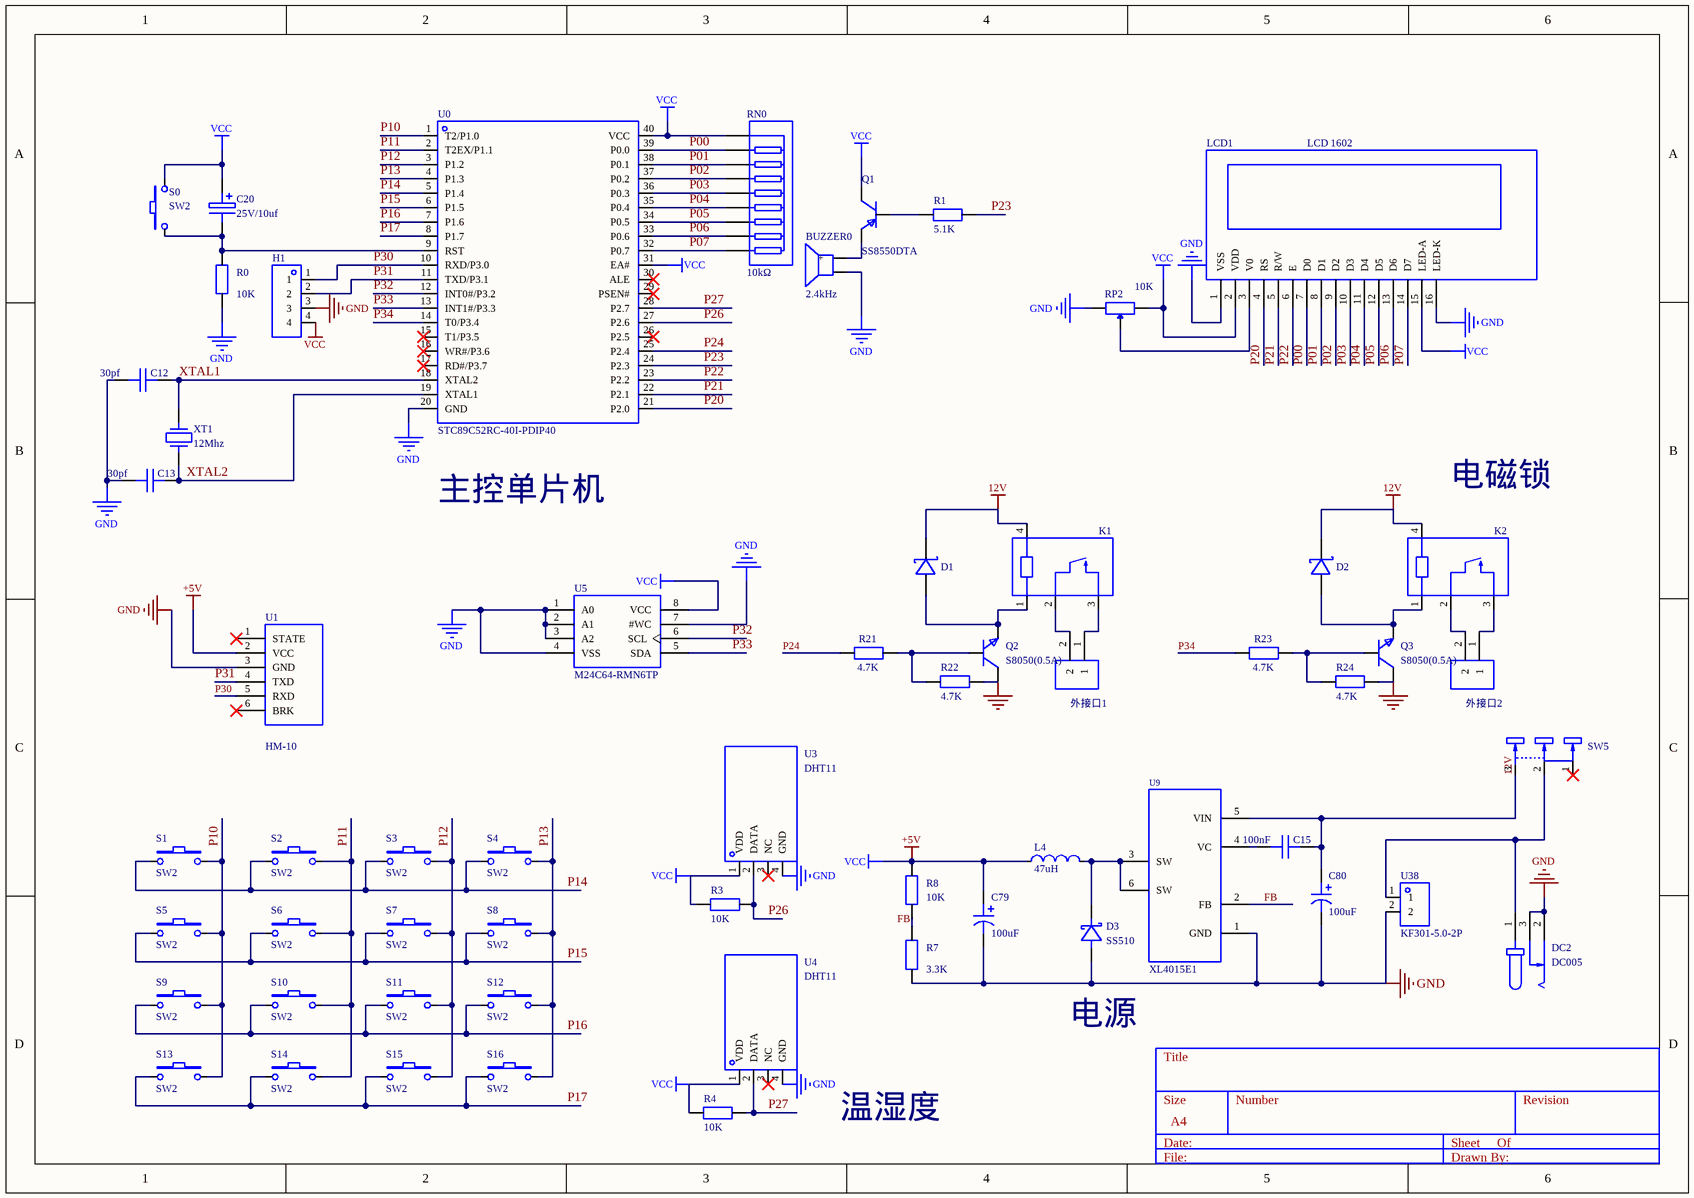
[diagram p0: MISC52141-3.schdoc]
# Altium project MISC52141-2.PrjPcb
1 sheet, 59 parts. Net scope: global (net labels, ports and power ports of the same name join across sheets).
Board file: MISC52141.pcbdoc

## Sheet MISC52141-3.schdoc
size 297 x 209 mm

### Parts
BUZZER0  2.4kHz  [BUZ-TH_BD12.0-P7.60-D0.6-FD]
C12  30pf  [C0805]
C13  30pf  [C0805]
C15  100nF  [C0805]
C20  value 25V/10uf  [CAP-TH_BD5.0-P2.00-D0.5-FD-A]  (hidden comment: CAP-E)
C79  100uF  [CAP-SMD_BD6.3-L6.6-W6.6-LS7.4-FD]
C80  100uF  [CAP-SMD_BD6.3-L6.6-W6.6-LS7.4-FD]
D1  (no value)  [SMC_L6.9-W5.9-LS7.9-RD]
D2  (no value)  [SMC_L6.9-W5.9-LS7.9-RD]
D3  SS510  [SMA_L4.3-W2.6-LS5.0-RD]
DC2  DC005  [DC-IN-TH_DC005]
H1  (no value)  [HDR-TH_4P-P2.54-V-F]
K1  (no value)  [RELAY-TH_G5NB-1A-E-DCXX]
K2  (no value)  [RELAY-TH_G5NB-1A-E-DCXX]
L4  47uH  [IND-SMD_L12.3-W12.3]
LCD1  LCD 1602  [LCD1602]
Q1  SS8550DTA  [TO-92-3_L4.8-W3.7-P2.54-L]
Q2  S8050(0.5A)  [SOT-23-3_L2.9-W1.3-P1.90-LS2.4-BR]
Q3  S8050(0.5A)  [SOT-23-3_L2.9-W1.3-P1.90-LS2.4-BR]
R0  10K  [R0805]
R1  5.1K  [R0805]
R3  10K  [R0805]
R4  10K  [R0805]
R7  3.3K  [R0805]
R8  10K  [R0805]
R21  4.7K  [R0805]
R22  4.7K  [R0805]
R23  4.7K  [R0805]
R24  4.7K  [R0805]
RN0  10kΩ  [RES-ARRAY-TH_9P-P2.54-D1.0]
RP2  10K  [RES-ADJ-TH_3296W-1-203]
S0  SW2  [SW-SMD_L3.9-W2.9-LS5.0]
S1  SW2  [SW-SMD_L3.9-W2.9-LS5.0]
S2  SW2  [SW-SMD_L3.9-W2.9-LS5.0]
S3  SW2  [SW-SMD_L3.9-W2.9-LS5.0]
S4  SW2  [SW-SMD_L3.9-W2.9-LS5.0]
S5  SW2  [SW-SMD_L3.9-W2.9-LS5.0]
S6  SW2  [SW-SMD_L3.9-W2.9-LS5.0]
S7  SW2  [SW-SMD_L3.9-W2.9-LS5.0]
S8  SW2  [SW-SMD_L3.9-W2.9-LS5.0]
S9  SW2  [SW-SMD_L3.9-W2.9-LS5.0]
S10  SW2  [SW-SMD_L3.9-W2.9-LS5.0]
S11  SW2  [SW-SMD_L3.9-W2.9-LS5.0]
S12  SW2  [SW-SMD_L3.9-W2.9-LS5.0]
S13  SW2  [SW-SMD_L3.9-W2.9-LS5.0]
S14  SW2  [SW-SMD_L3.9-W2.9-LS5.0]
S15  SW2  [SW-SMD_L3.9-W2.9-LS5.0]
S16  SW2  [SW-SMD_L3.9-W2.9-LS5.0]
SW5  SS-12D10L5  [SW-TH_SS-12D10L5]  (value not drawn)
U0  STC89C52RC-40I-PDIP40  [DIP-40_L52.0-W13.7-P2.54-LS15.2-BL]
U1  HM-10  [HM-10.288]
U3  DHT11  [SENSOR-TH_DHT11]
U4  DHT11  [SENSOR-TH_DHT11]
U5  M24C64-RMN6TP  [SOIC-8_L5.0-W4.0-P1.27-LS6.0-BL]
U9  XL4015E1  [TO-263-5_L10.2-W8.9-P1.70-TL]
U38  KF301-5.0-2P  [CONN-TH_P5.00_KF301-5.0-2P]
XT1  value 12Mhz  [HC-49S_L7.2-W3.2]  (hidden comment: XT)
外接口1  (no value)  [CONN-TH_2P-P5.00_WJ500V-5.08-2P]
外接口2  (no value)  [CONN-TH_2P-P5.00_WJ500V-5.08-2P]

### Nets
12V: C15.1 C80.1 D1.1(C) D2.1(C) K1.4 K2.4 SW5.3 U9.5(VIN)
+5V: C20.1 C79.1 H1.4 L4.1 LCD1.2(VDD) LCD1.15(LED-A) Q1.3(C) R3.2 R4.2 R8.2 RN0.1 RP2.1 S0.2 U0.31(EA#) U0.40(VCC) U1.2(VCC) U3.1(VDD) U4.1(VDD) U5.8(VCC)  [also labelled VCC]
GND: BUZZER0.2 C12.2 C13.2 C79.2 C80.2 D3.2(A) DC2.2 DC2.3 H1.3 LCD1.1(VSS) LCD1.16(LED-K) Q2.3(C) Q3.3(C) R0.1 R7.1 R22.1 R24.1 RP2.3 U0.20(GND) U1.3(GND) U3.4(GND) U4.4(GND) U5.1(A0) U5.2(A1) U5.3(A2) U5.4(VSS) U5.7(#WC) U9.1(GND) U38.2
FB: R7.2 R8.1 U9.2(FB)
P00: LCD1.7(D0) RN0.2 U0.39(P0.0)
P01: LCD1.8(D1) RN0.3 U0.38(P0.1)
P02: LCD1.9(D2) RN0.4 U0.37(P0.2)
P03: LCD1.10(D3) RN0.5 U0.36(P0.3)
P04: LCD1.11(D4) RN0.6 U0.35(P0.4)
P05: LCD1.12(D5) RN0.7 U0.34(P0.5)
P06: LCD1.13(D6) RN0.8 U0.33(P0.6)
P07: LCD1.14(D7) RN0.9 U0.32(P0.7)
P10: S1.2 S5.2 S9.2 S13.2 U0.1(T2/P1.0)
P11: S2.2 S6.2 S10.2 S14.2 U0.2(T2EX/P1.1)
P12: S3.2 S7.2 S11.2 S15.2 U0.3(P1.2)
P13: S4.2 S8.2 S12.2 S16.2 U0.4(P1.3)
P14: S1.1 S2.1 S3.1 S4.1 U0.5(P1.4)
P15: S5.1 S6.1 S7.1 S8.1 U0.6(P1.5)
P16: S9.1 S10.1 S11.1 S12.1 U0.7(P1.6)
P17: S13.1 S14.1 S15.1 S16.1 U0.8(P1.7)
P20: LCD1.4(RS) U0.21(P2.0)
P21: LCD1.5(R/W) U0.22(P2.1)
P22: LCD1.6(E) U0.23(P2.2)
P23: R1.1 U0.24(P2.3)
P24: R21.2 U0.25(P2.4)
P26: R3.1 U0.27(P2.6) U3.2(DATA)
P27: R4.1 U0.28(P2.7) U4.2(DATA)
P30: H1.1 U0.10(RXD/P3.0) U1.5(RXD)
P31: H1.2 U0.11(TXD/P3.1) U1.4(TXD)
P32: U0.12(INT0#/P3.2) U5.6(SCL)
P33: U0.13(INT1#/P3.3) U5.5(SDA)
P34: R23.2 U0.14(T0/P3.4)
XTAL1: C12.1 U0.18(XTAL2) XT1.2
XTAL2: C13.1 U0.19(XTAL1) XT1.1
NetBUZZER0_1: BUZZER0.1(+) Q1.1(E)
NetC15_2: C15.2 U9.4(VC)
NetC20_2: C20.2 R0.2 S0.1 U0.9(RST)
NetD1_2: D1.2(A) K1.1 Q2.2(E)
NetD2_2: D2.2(A) K2.1 Q3.2(E)
NetD3_1: D3.1(K) L4.2 U9.3(SW) U9.6(SW)
NetDC2_1: DC2.1 SW5.2 U38.1
NetK1_2: K1.2 外接口1.2
NetK1_3: K1.3 外接口1.1
NetK2_2: K2.2 外接口2.2
NetK2_3: K2.3 外接口2.1
NetLCD1_3: LCD1.3(V0) RP2.2
NetQ1_2: Q1.2(B) R1.2
NetQ2_1: Q2.1(B) R21.1 R22.2
NetQ3_1: Q3.1(B) R23.1 R24.2

Not connected (* = marked no-connect by the designer): SW5 1*; U0 15(T1/P3.5)* 16(WR#/P3.6)* 17(RD#/P3.7)* 26(P2.5)* 29(PSEN#)* 30(ALE)*; U1 1(STATE)* 6(BRK)*; U3 3(NC)*; U4 3(NC)*

### Notes on the sheet
- 主控单片机
- (near K2) 电磁锁
- (near D3) 电源
- 温湿度
- Title
- File:
- Date:
- Size
- A4
- Number
- Drawn By:
- Sheet
- Of
- Revision

### Library data of the parts
BUZZER0 = TMB12A05_C96093: 驱动方式:有源(内含驱动线路);构造类型:电磁式;额定电压:5V;频率:2.4kHz;声压(SPL):85dB;; Manufacturer: 华能; AddInBom: yes; ModelId: 16ab50e14c5b4f2c986c135bdba60e370819f05c4eef4c71ace90d822a990e87; ModelName: BUZ-TH_D12.0-H9.5-P7.60; ModelTransform: 472.44,472.176,0,90,0,0,-0.787,0,-177.165; Voltage Rating: 5V; Voltage - Supply: 4V~8V; Current Consumption: 30mA; Sound Pressure Level(SPL): 85dB; Symbol: TMB12A05; Device: TMB12A05_C96093; LCSC Part Name: 有源(内含驱动线路) 电磁式 2.4kHz; SupplierPart: C96093; ManufacturerPart: TMB12A05; Supplier Footprint: 插件,D=12mm; JLCPCB Part Class: Extended Part; Datasheet: https://item.szlcsc.com/datasheet/TMB12A05/97297.html; Supplier: LCSC; ConvertToPcb: yes; FootprintName: BUZ-TH_BD12.0-P7.60-D0.6-FD; Driver Circuitry: 有源(内含驱动线路); Technology: 电磁式; Value: 2.4kHz; Diameter(φD): 12mm; Length: -; Width: -; Height: 9.8mm; Operating Temperature: -40℃~+85℃
C12 C13 C15 = CAP_0805: Symbol: CapAcitance; 3D Model: 1ba041120af144c991958decab20d241; 3D Model Transform: 78.74,51.181,0,0,0,0,0,0.0005,0; ConvertToPcb: yes; ModelName: C0805_L2.0-W1.3-H1.3; Device: CAP_0805; Supplier Footprint: 0805; AddInBom: yes; FootprintName: C0805
  C12 C13: Value: 30pf
  C15: Value: 100nF
C20 = CAP-E: 电解电容; Origin Footprint 1: RB.1/.22(6.35); Origin Footprint 2: CAPSO_5*7; Origin Footprint 3: CAPSO_10*10; Origin Footprint 4: capso_5*5; Origin Footprint 5: capso_8*10; Origin Footprint 6: RB.1/.2; Origin Footprint 7: RB.3/.6; Origin Footprint 8: RB.3/.7; Origin Footprint 9: RB.4/.8; Origin Footprint 10: RB.5/1.0; Origin Footprint 11: RB.1/.25(8.04); Origin Footprint 12: RB.2/.4(10.13); Origin Footprint 13: RB.2/.5(13.05); AddInBom: yes; Device: CAP-E; Symbol: CAP-E; Design Item ID: CAP-E; Library Name: 新原理图库; ConvertToPcb: yes
C79 C80 = RVT100UF35V67RV0034: 容值:100uF;精度:±20%;额定电压:35V;纹波电流:87mA@120kHz;等效串联电阻:-;; Manufacturer: KNSCHA(科尼盛); 3D Model: 1416614ffc1f4b92814ec0fcf834cf2d; 3D Model Transform: 291.338,259.842,0,180,0,0,-0.004,-0.007,0; Tolerance: ±20%; Rated Voltage: 35V; φD: 6.3mm; L: 7.7mm; Lifetime @ Temp: 2000hrs@105℃; AddInBom: yes; Symbol: RVT100UF35V67RV0034; Device: RVT100UF35V67RV0034; LCSC Part Name: 100uF ±20% 35V; Supplier Footprint: SMD,D6.3xL7.7mm; Datasheet: https://atta.szlcsc.com/upload/public/pdf/source/20210528/C2836442_7F6389BF36F63F32D6DF3A507E8E95D6.pdf; Ripple Current: 87mA@120kHz; Equivalent Series Resistance(ESR): -; Operating Temperature: -55℃~+105℃; Supplier: LCSC; Supplier Part: C2836442; Manufacturer Part: RVT100UF35V67RV0034; Value: 100uF; JLCPCB Part Class: 扩展库; ConvertToPcb: yes; FootprintName: CAP-SMD_BD6.3-L6.6-W6.6-LS7.4-FD; ModelName: CAP-SMD_BD6.3-L6.6-W6.6-LS7.4-FD
D1 D2 = SS34_C154551: 3D Model: 4f14ab132b494223bc17c7f39616ac35; 3D Model Transform: 314.96,236.22,0,0,0,0,0,0,0; AddInBom: yes; Symbol: SS34_C154551; Device: SS34_C154551; ConvertToPcb: yes; FootprintName: SMC_L6.9-W5.9-LS7.9-RD; ModelName: SMC_L6.9-W5.9-LS7.9-RD
D3 = SS510_C727067: 二极管配置:独立式;直流反向耐压(Vr):100V;平均整流电流(Io):5A;正向压降(Vf):850mV@5A;; Manufacturer: TWGMC(台湾迪嘉); 3D Model: c45541be4ee342138706b28195cdf845; 3D Model Transform: 196.85,102.362,0,0,0,0,0,0,0; Diode Configuration: 独立式; Reverse Voltage (Vr): 100V; Average Rectified Current (Io): 5A; Reverse Leakage Current (Ir): 500uA@100V; AddInBom: yes; Symbol: SS510_C727067; Device: SS510_C727067; LCSC Part Name: 电压:100V 电流:5A; Supplier Footprint: SMA(DO-214AC); Datasheet: https://atta.szlcsc.com/upload/public/pdf/source/20200828/C727064_BD0A2B36CBC76CEA4B6710C57718D41F.pdf; Forward Voltage (Vf@If): 850mV@5A; Supplier: LCSC; Supplier Part: C727067; Manufacturer Part: SS510; JLCPCB Part Class: 扩展库; ConvertToPcb: yes; FootprintName: SMA_L4.3-W2.6-LS5.0-RD; ModelName: SMA_L4.3-W2.6-LS5.0-RD
DC2 = DC005: 连接器类型:DC电源插座;安装方式:弯插;触点内径:2mm;触点外径:6.3mm;额定电流:500mA;额定电压:12V;工作温度:-30℃~+70℃;; Manufacturer: SHOU HAN(首韩); Symbol: DC005_C431533; 3D Model: f168fe383f964e0ea2af0127ff6ac7b40819f05c4eef4c71ace90d822a990e87; 3D Model Transform: 366.141,553.149,0,270,0,0,-141.734,88.583,-149.606; Connector Type: DC电源插座; Inside Contact Diameter: 2mm; Outside Contact Diameter: 6.3mm; Current Rating: 500mA; Voltage Rating (Max): 12V; AddInBom: yes; Device: DC005; LCSC Part Name: DC005-2.0 黑（铁）; Supplier Part: C431533; Manufacturer Part: DC005; Supplier Footprint: 插件; JLCPCB Part Class: Extended Part; Datasheet: https://item.szlcsc.com/datasheet/DC005/427890.html; Supplier: LCSC; Mounting Type: 弯插; Operating Temperature: -30℃~+70℃; ConvertToPcb: yes; FootprintName: DC-IN-TH_DC005; ModelName: DC-IN-TH_DC005
H1 = HDR-F_2.54_1x4P: Symbol: 2.54-1*4P母; ConvertToPcb: yes; ModelId: d187812051054f85879fcaa51a310d8e0819f05c4eef4c71ace90d822a990e87; ModelTransform: 419.6842,98.464,0,0,0,0,0,0,-118.11; Device: HDR-F_2.54_1x4P; AddInBom: yes; SupplierPart: C2718488; Supplier Footprint: 插件; FootprintName: HDR-TH_4P-P2.54-V-F; ModelName: HDR-TH_4P-P2.54-V-F
K1 K2 = G5NB-1A-E-12VDC: 3D Model: 6120fb8104464971ad0bbab563986a92; 3D Model Transform: 807.085,275.984,0,0,0,0,-0.002,-0.001,-118.11; AddInBom: yes; ModelName: RELAY-TH_L20.5-W7.0-H15.0; Symbol: G5NB-1A-E-12VDC; Device: G5NB-1A-E-12VDC; ConvertToPcb: yes; FootprintName: RELAY-TH_G5NB-1A-E-DCXX
L4 = SMDRI127-470MT: 类型:屏蔽电感;电感值:47uH;精度:±20%;额定电流:2.5A;饱和电流(Isat):4.6A;; Manufacturer: SXN(顺翔诺); 3D Model: 1430fda232714ed3b12b8476f42d35be; 3D Model Transform: 494.75925,492.125,0,0,0,0,-0.005,0,0; Type: 屏蔽电感; Tolerance: ±20%; Rated Current: 2.5A; Saturation Current (Isat): 4.6A; DC Resistance (DCR): 100mΩ; AddInBom: yes; ModelName: SMD-PIND_L12.5-W12.5-H8.0; Symbol: SMDRI127-470MT; Device: SMDRI127-470MT; LCSC Part Name: 47uH ±20% 4.6A; Supplier Footprint: SMD; Datasheet: https://atta.szlcsc.com/upload/public/pdf/source/20210810/6F96FDC19AA308DD2AD166FFB9640E87.pdf; Supplier: LCSC; Manufacturer Part: SMDRI127-470MT; Value: 47uH; Supplier Part: C9906; JLCPCB Part Class: 扩展库; ConvertToPcb: yes; FootprintName: IND-SMD_L12.3-W12.3
LCD1 = LCD 1602: AddInBom: yes; Origin Footprint: LCD-1602; Device: LCD 1602; Symbol: LCD 1602; Design Item ID: LCD 1602; Library Name: MadeSchlibS; BOM名称: LCD 1602; Description: LCD 1602; ConvertToPcb: yes
Q1 = SS8550DTA: 晶体管类型:PNP;集电极电流(Ic):1.5A;集射极击穿电压(Vceo):25V;耗散功率(Pd):2W;直流电流增益(hFE):40@800mA,1V;; Manufacturer: onsemi(安森美); Add into BOM: yes; 3D Model: 9cd5952e07174348a2979f24811496f3; 3D Model Transform: 218.1098,145.669,0,0,0,0,0,13.78,-137.795; type: PNP; Current - Collector(Ic): 1.5A; Collector - Emitter Voltage VCEO: 25V; Pd - Power Dissipation: 2W; Transition frequency(fT): 100MHz; Current - Collector Cutoff: 100nA; Vce Saturation(VCE(sat)): 280mV@800mA,80mA; ModelName: TO-92-3_L4.8-W3.7-H4.8-P2.54; Symbol: SS8550DTA; Device: SS8550DTA; Convert to PCB: yes; LCSC Part Name: PNP 电流:1.5A 电压:25V; Supplier Part: C903228; Manufacturer Part: SS8550DTA; Supplier Footprint: TO-92-3; JLCPCB Part Class: Extended Part; Datasheet: https://item.szlcsc.com/datasheet/SS8550DTA/968666.html; Supplier: LCSC; DC Current Gain: 40@800mA,1V; Operating Temperature: -65℃~+150℃; FootprintName: TO-92-3_L4.8-W3.7-P2.54-L
Q2 Q3 = S8050(0.5A): 晶体管类型:NPN;集电极电流(Ic):500mA;集射极击穿电压(Vceo):25V;耗散功率(Pd):300mW;直流电流增益(hFE):120;; Manufacturer: EIC; 3D Model: c62791f0466c4ae2a892c056b845b0ca0819f05c4eef4c71ace90d822a990e87; 3D Model Transform: 98.425,114.173,0,180,0,0,0.0005,-0.0005,0; type: NPN; Current - Collector(Ic): 500mA; Collector - Emitter Voltage VCEO: 25V; Pd - Power Dissipation: 300mW; DC Current Gain: 120; Transition frequency(fT): 150MHz; Current - Collector Cutoff: 100nA; Vce Saturation(VCE(sat)): 600mV; Emitter-Base Voltage(Vebo): 5V; Number: 1个NPN; AddInBom: yes; ModelName: SOT-23-3P_L2.9-W1.3-H1.0-LS2.4-P0.95; Symbol: S8050(0.5A); Device: S8050(0.5A); LCSC Part Name: 电流:0.5A 电压:25V; Supplier Part: C3014350; Manufacturer Part: S8050(0.5A); Supplier Footprint: SOT-23; JLCPCB Part Class: Extended Part; Datasheet: https://item.szlcsc.com/datasheet/S8050(0.5A)/3524496.html; Supplier: LCSC; ConvertToPcb: yes; FootprintName: SOT-23-3_L2.9-W1.3-P1.90-LS2.4-BR
R0 R1 R3 R4 R7 R8 R21-R24 = Res_0805: Symbol: 电阻; 3D Model: 37a81e68749a4138bd2dfa6897b24b85; 3D Model Transform: 78.74,51.181,0,0,0,0,0,-0.0005,0; ConvertToPcb: yes; ModelName: R0805_L2.0-W1.3-H0.6; Device: Res_0805; AddInBom: yes; FootprintName: R0805
  R0 R3 R4: Value: 10K; Supplier Footprint: 0805
  R1: Value: 5.1K; Supplier Footprint: 0805
  R7: Value: 3.3K; Supplier Footprint: 0805
  R8: Supplier Footprint: 0805; Value: 10K
  R21-R24: Value: 4.7K
RN0 = A09-103JP: 电阻器数:8;阻值:10kΩ;精度:±5%;单个元件功率:125mW;温度系数:±100ppm/℃;; Manufacturer: FH(风华); AddInBom: yes; ModelId: d106c67f29e14d8080ba548247a719a10819f05c4eef4c71ace90d822a990e87; ModelName: SIP-9_L22.8-W3.0-H8.5-P2.54; ModelTransform: 918.1084,118.11,0,0,0,0,0,0,-137.795; Number of Resistors: 8; Tolerance: ±5%; Power(Watts): 125mW; Symbol: A09-103JP; Device: A09-103JP; LCSC Part Name: 10kΩ ±5%; SupplierPart: C8692; ManufacturerPart: A09-103JP; Supplier Footprint: SIP-9-2.54mm; JLCPCB Part Class: Extended Part; Datasheet: https://atta.szlcsc.com/upload/public/pdf/source/20181127/C336620_2E84FA9E7B5BF76546BC661699514FB8.pdf; Supplier: LCSC; ConvertToPcb: yes; FootprintName: RES-ARRAY-TH_9P-P2.54-D1.0; Value: 10kΩ; Temperature Coefficient: ±100ppm/℃; Number of Pins: 9
RP2 = 10K: 插件单联电位器; Origin Footprint 1: 3296W; Symbol: RP-ID; BOM名称: 插件电位器; Origin Footprint 2: 3306W; Origin Footprint 3: 3319P; Origin Footprint 4: 3362P; Origin Footprint 5: 3386W; Origin Footprint 6: RM065; Origin Footprint 7: WH148-1-G15; Origin Footprint 8: WH148-1-G18; Origin Footprint 9: WH148-1-G20; Origin Footprint 10: WH148-1-G25; Origin Footprint 11: 3266W; Origin Footprint 12: 3266X; Origin Footprint 13: 3266Y; Origin Footprint 14: 3266Z; Origin Footprint 15: XV09223NPV-20F; Origin Footprint 16: XV09223NPV-25F; Origin Footprint 17: XV09223NPV-30F; Origin Footprint 18: 3006P; AddInBom: yes; ModelId: b182808559bb43bda9e7de64b64134cb; Device: 10K; Design Item ID: RP-ID; Library Name: MadeSchlibS; ConvertToPcb: yes; ModelName: 3296W
S0 = SW2: Origin Footprint 1: SW-4; Origin Footprint 3: key-3-5p; Origin Footprint 4: SW-PB2; Origin Footprint 5: SW-6-1; AddInBom: yes; Device: SW2; Symbol: SW2; Design Item ID: SW2; Library Name: 新原理图库; Origin Footprint 2: SW2; ConvertToPcb: yes
S1 = SW2: Origin Footprint 1: SW-4; Origin Footprint 3: key-3-5p; Origin Footprint 4: SW-PB2; Origin Footprint 5: SW-6-1; UniqueId: 0ac0bd892f9b1ec0; AddInBom: yes; Device: SW2; Symbol: SW2; Design Item ID: SW2; Library Name: 新原理图库; Origin Footprint 2: SW2; ConvertToPcb: yes
S2 = SW2: Origin Footprint 1: SW-4; Origin Footprint 3: key-3-5p; Origin Footprint 4: SW-PB2; Origin Footprint 5: SW-6-1; UniqueId: 16ca49f37df57620; AddInBom: yes; Device: SW2; Symbol: SW2; Design Item ID: SW2; Library Name: 新原理图库; Origin Footprint 2: SW2; ConvertToPcb: yes
S3 = SW2: Origin Footprint 1: SW-4; Origin Footprint 3: key-3-5p; Origin Footprint 4: SW-PB2; Origin Footprint 5: SW-6-1; UniqueId: b21ed8cc1c3b642b; AddInBom: yes; Device: SW2; Symbol: SW2; Design Item ID: SW2; Library Name: 新原理图库; Origin Footprint 2: SW2; ConvertToPcb: yes
S4 = SW2: Origin Footprint 1: SW-4; Origin Footprint 3: key-3-5p; Origin Footprint 4: SW-PB2; Origin Footprint 5: SW-6-1; UniqueId: b4af5bc4dd85243d; AddInBom: yes; Device: SW2; Symbol: SW2; Design Item ID: SW2; Library Name: 新原理图库; Origin Footprint 2: SW2; ConvertToPcb: yes
S5 = SW2: Origin Footprint 1: SW-4; Origin Footprint 3: key-3-5p; Origin Footprint 4: SW-PB2; Origin Footprint 5: SW-6-1; UniqueId: b2403b9688924408; AddInBom: yes; Device: SW2; Symbol: SW2; Design Item ID: SW2; Library Name: 新原理图库; Origin Footprint 2: SW2; ConvertToPcb: yes
S6 = SW2: Origin Footprint 1: SW-4; Origin Footprint 3: key-3-5p; Origin Footprint 4: SW-PB2; Origin Footprint 5: SW-6-1; UniqueId: 30ed59e7372531b3; AddInBom: yes; Device: SW2; Symbol: SW2; Design Item ID: SW2; Library Name: 新原理图库; Origin Footprint 2: SW2; ConvertToPcb: yes
S7 = SW2: Origin Footprint 1: SW-4; Origin Footprint 3: key-3-5p; Origin Footprint 4: SW-PB2; Origin Footprint 5: SW-6-1; UniqueId: 645ed82ea5a47d74; AddInBom: yes; Device: SW2; Symbol: SW2; Design Item ID: SW2; Library Name: 新原理图库; Origin Footprint 2: SW2; ConvertToPcb: yes
S8 = SW2: Origin Footprint 1: SW-4; Origin Footprint 3: key-3-5p; Origin Footprint 4: SW-PB2; Origin Footprint 5: SW-6-1; UniqueId: 528eaac5fe170b76; AddInBom: yes; Device: SW2; Symbol: SW2; Design Item ID: SW2; Library Name: 新原理图库; Origin Footprint 2: SW2; ConvertToPcb: yes
S9 = SW2: Origin Footprint 1: SW-4; Origin Footprint 3: key-3-5p; Origin Footprint 4: SW-PB2; Origin Footprint 5: SW-6-1; UniqueId: 82f79cc1abfd6827; AddInBom: yes; Device: SW2; Symbol: SW2; Design Item ID: SW2; Library Name: 新原理图库; Origin Footprint 2: SW2; ConvertToPcb: yes
S10 = SW2: Origin Footprint 1: SW-4; Origin Footprint 3: key-3-5p; Origin Footprint 4: SW-PB2; Origin Footprint 5: SW-6-1; UniqueId: 8a04837b5e6de309; AddInBom: yes; Device: SW2; Symbol: SW2; Design Item ID: SW2; Library Name: 新原理图库; Origin Footprint 2: SW2; ConvertToPcb: yes
S11 = SW2: Origin Footprint 1: SW-4; Origin Footprint 3: key-3-5p; Origin Footprint 4: SW-PB2; Origin Footprint 5: SW-6-1; UniqueId: 6714c845c0bfadd2; AddInBom: yes; Device: SW2; Symbol: SW2; Design Item ID: SW2; Library Name: 新原理图库; Origin Footprint 2: SW2; ConvertToPcb: yes
S12 = SW2: Origin Footprint 1: SW-4; Origin Footprint 3: key-3-5p; Origin Footprint 4: SW-PB2; Origin Footprint 5: SW-6-1; UniqueId: b0f51aaad8bcaf38; AddInBom: yes; Device: SW2; Symbol: SW2; Design Item ID: SW2; Library Name: 新原理图库; Origin Footprint 2: SW2; ConvertToPcb: yes
S13 = SW2: Origin Footprint 1: SW-4; Origin Footprint 3: key-3-5p; Origin Footprint 4: SW-PB2; Origin Footprint 5: SW-6-1; UniqueId: 992e87e878284c83; AddInBom: yes; Device: SW2; Symbol: SW2; Design Item ID: SW2; Library Name: 新原理图库; Origin Footprint 2: SW2; ConvertToPcb: yes
S14 = SW2: Origin Footprint 1: SW-4; Origin Footprint 3: key-3-5p; Origin Footprint 4: SW-PB2; Origin Footprint 5: SW-6-1; UniqueId: 2d0f9b3bdc334ecd; AddInBom: yes; Device: SW2; Symbol: SW2; Design Item ID: SW2; Library Name: 新原理图库; Origin Footprint 2: SW2; ConvertToPcb: yes
S15 = SW2: Origin Footprint 1: SW-4; Origin Footprint 3: key-3-5p; Origin Footprint 4: SW-PB2; Origin Footprint 5: SW-6-1; UniqueId: d9b92ad1e11f2f39; AddInBom: yes; Device: SW2; Symbol: SW2; Design Item ID: SW2; Library Name: 新原理图库; Origin Footprint 2: SW2; ConvertToPcb: yes
S16 = SW2: Origin Footprint 1: SW-4; Origin Footprint 3: key-3-5p; Origin Footprint 4: SW-PB2; Origin Footprint 5: SW-6-1; UniqueId: efb94aec797f6b83; AddInBom: yes; Device: SW2; Symbol: SW2; Design Item ID: SW2; Library Name: 新原理图库; Origin Footprint 2: SW2; ConvertToPcb: yes
SW5 = SS-12D10L5: 电路结构:单刀双掷;安装方式:直插;开关颜色:黑色;额定电流:3A;额定电压:125V;工作寿命:1万次;; Manufacturer: XKB Connection(中国星坤); 3D Model: c49f07a32c154ec8ad7cf47670a539810819f05c4eef4c71ace90d822a990e87; 3D Model Transform: 511.81394,267.716,0,0,0,0,0,0,-220.472; Circuit: 单刀双掷; Actuator Style: 矩形柱状; Switch Height: 6.4mm; Actuator Color: 黑色; Current Rating: 3A; Voltage Rating: 125V; Life: 1万次; AddInBom: yes; ModelName: SW-TH_L13.0-W6.8-H6.4-P4.7; Symbol: SS-12D10L5; Device: SS-12D10L5; LCSC Part Name: 柄长5mm 直插双档 滑动开关; Supplier Part: C319012; Manufacturer Part: SS-12D10L5; Supplier Footprint: 插件,13x6.8mm; JLCPCB Part Class: Extended Part; Datasheet: https://item.szlcsc.com/datasheet/SS-12D10L5/300104.html; Supplier: LCSC; Termination Style: PC引脚; Length: 13mm; Width: 6.8mm; Mounting Type: 直插; Operating Temperature: -40℃~+85℃; ConvertToPcb: yes; FootprintName: SW-TH_SS-12D10L5
U0 = STC89C52RC-40I-PDIP40: CPU内核:51家族;CPU最大主频:-;; Manufacturer: STC; AddInBom: yes; ModelId: 16d4686a009b4ddca948f91eddb57b140819f05c4eef4c71ace90d822a990e87; ModelName: DIP-40_L52.3-W13.8-H4.0-LS15.24-P2.54; ModelTransform: 2059.051,615.743,0,0,0,0,0,0,-118.11; CPU Core: 51家族; Program Storage Size: 8KB; Program Memory Type: FLASH; Voltage - Supply: 3.3V~5.5V; Symbol: STC89C52RC-40I; Device: STC89C52RC-40I-PDIP40; LCSC Part Name: 单片机原理及应用; SupplierPart: C14022; ManufacturerPart: STC89C52RC-40I-PDIP40; Supplier Footprint: DIP-40; JLCPCB Part Class: Extended Part; Datasheet: https://item.szlcsc.com/datasheet/STC89C52RC-40I-PDIP40/14679.html; Supplier: LCSC; ConvertToPcb: yes; FootprintName: DIP-40_L52.0-W13.7-P2.54-LS15.2-BL; CPU Maximum Speed: -; RAM Size: -; EEPROM: -; Number of I/O: -; ADC (Bit): -; DAC (Bit): -
U1 = hm10: 蓝牙; Convert to PCB: yes; Symbol: hm10; Device: hm10; FootprintName: HM-10.288; AddInBom: yes
U3 U4 = DHT11: 温度范围:-20℃~+60℃;湿度范围:5%RH~95%RH;湿度精度:±5%RH;; Manufacturer: 广州奥松; AddInBom: yes; ModelId: 6dde47d4d8bf4fa598dffcc067449c1d0819f05c4eef4c71ace90d822a990e87; ModelTransform: 236.25937,492.125,0,270,0,0,0,-11.811,-196.85; Voltage - Supply: 3.3V~5.5V; Current - Supply: 1mA; Humidity Tolerance: ±5%RH; Temperature Tolerance: ±2℃; Symbol: DHT11; Device: DHT11; LCSC Part Name: 新款电容式数字温湿度传感器,老款已停产16.1x12.6x5.8mm DHT11  电容式传感器; SupplierPart: C117051; ManufacturerPart: DHT11; Supplier Footprint: SIP-4; JLCPCB Part Class: Extended Part; Datasheet: https://item.szlcsc.com/datasheet/DHT11/118309.html; Supplier: LCSC; ConvertToPcb: yes; FootprintName: SENSOR-TH_DHT11; ModelName: SENSOR-TH_DHT11; Temperature Range: -20℃~+60℃; Humidity: 5%RH~95%RH
U5 = M24C64-RMN6TP: 接口类型:I2C;存储容量:64Kbit;时钟频率(fc):1MHz;; Manufacturer: ST(意法半导体); AddInBom: yes; ModelId: 7abc64c95a1a4a04a4ef38f9097c870b0819f05c4eef4c71ace90d822a990e87; ModelTransform: 192.913,236.22,0,0,0,0,0,0,0; Interface: I2C; Memory Size: 64Kbit; Clock Frequency: 1MHz; Voltage - Supply: 1.8V~5.5V; Write Cycle Time(Tw): 5ms; Data Retention - TDR (Year): 200年; Write Cycle Endurance: 400万次; Symbol: M24C64-RMN6TP; Device: M24C64-RMN6TP; LCSC Part Name: 64 Kbit串行I2C总线EEPROM; SupplierPart: C79988; ManufacturerPart: M24C64-RMN6TP; Supplier Footprint: SOIC-8; JLCPCB Part Class: Extended Part; Datasheet: https://item.szlcsc.com/datasheet/M24C64-RMN6TP/81133.html; Supplier: LCSC; ConvertToPcb: yes; FootprintName: SOIC-8_L5.0-W4.0-P1.27-LS6.0-BL; ModelName: SOIC-8_L5.0-W4.0-P1.27-LS6.0-BL; Operating Temperature: -40℃~+85℃
U9 = XL4015E1: 功能类型:降压型;输入电压:-;输出电流(最大值):-;; Manufacturer: XLSEMI(芯龙); 3D Model: 4e421a816a7f4d57b8710832ddea550a; 3D Model Transform: 401.574,560.17797,0,270,0,0,62.156,-0.08,0; Function: 降压型; AddInBom: yes; ModelName: TO-263-5-5P_L10.2-W8.7-H4.5-LS14.4-P1.70; Symbol: XL4015E1; Device: XL4015E1; LCSC Part Name: XL4015E1; Supplier Footprint: TO-263-5; Datasheet: https://atta.szlcsc.com/upload/public/pdf/source/20150618/1457707323461.pdf; Synchronous Rectification: -; Number of Outputs: -; Topology: -; Input Voltage: -; Output Current (Max): -; Switching Frequency: -; Supplier: LCSC; Manufacturer Part: XL4015E1; Supplier Part: C51661; JLCPCB Part Class: 扩展库; ConvertToPcb: yes; FootprintName: TO-263-5_L10.2-W8.9-P1.70-TL
U38 = KF301-5.0-2P: 结构:1x2P;间距:5mm;颜色:蓝色;安装方式:直插;额定电流:17A;额定电压:250V;排数:1;线规 - AWG:14~22;线规 - 平方毫米:1.5;每排PIN数:2;工作温度范围:-30℃~+120℃;; Manufacturer: KEFA(科发); 3D Model: ccfba28652874fb7a69eea8ba34eb61b; 3D Model Transform: 417.322,299.21594,0,0,0,0,11.811,7.874,-137.795; Pitch: 5mm; Number of PINs Per Row: 2; Voltage Rating (Max): 250V; Wire Gauge - AWG: 14~22; Wire Gauge - mm2: 1.5; Structure: 1x2P; Current Rating (Max): 17A; AddInBom: yes; Symbol: KF301-5.0-2P; Device: KF301-5.0-2P; LCSC Part Name: 5mm 1x2P 排数:1 每排P数:2 直插; Supplier Part: C474881; Manufacturer Part: KF301-5.0-2P; Supplier Footprint: 插件,P=5mm; JLCPCB Part Class: 扩展库; Datasheet: https://atta.szlcsc.com/upload/public/pdf/source/20230317/03A5B5FC229D6F9225E8F51DA1A4E80A.pdf; Supplier: LCSC; Color: 蓝色; Number of Pins: 2P; Number of Rows: 1; Mounting Style: 直插; Operating Temperature Range: -30℃~+120℃; Number of Positions or Pins: 1x2P; Mounting Type: 直插; Current Rating: 17A; Operating Temperature: -30℃~+120℃; ConvertToPcb: yes; FootprintName: CONN-TH_P5.00_KF301-5.0-2P; ModelName: CONN-TH_P5.00_KF301-5.0-2P
XT1 = XT: 晶振; Origin Footprint 1: XTAL-D; Origin Footprint 2: XTAL-B; Origin Footprint 3: XTAL-NS; Origin Footprint 4: X5032; Origin Footprint 5: X5070; Origin Footprint 6: X6035; Origin Footprint 7: XTAL-4S8; Origin Footprint 8: XTAL32 - tie; Origin Footprint 9: XTAL; AddInBom: yes; Device: XT; Symbol: XT; Design Item ID: XT; Library Name: 新原理图库; ConvertToPcb: yes
外接口1 外接口2 = WJ500V-5.08-2P: Symbol: WJ500V-5.08-2P-14-00A; 3D Model: 0f4a503c8d3b4ae19ed61267f5e9a1d7; 3D Model Transform: 423.621,393.7,0,0,0,0,-11.811,19.685,-137.795; AddInBom: yes; Device: WJ500V-5.08-2P; ConvertToPcb: yes; FootprintName: CONN-TH_2P-P5.00_WJ500V-5.08-2P; ModelName: CONN-TH_2P-P5.00_WJ500V-5.08-2P